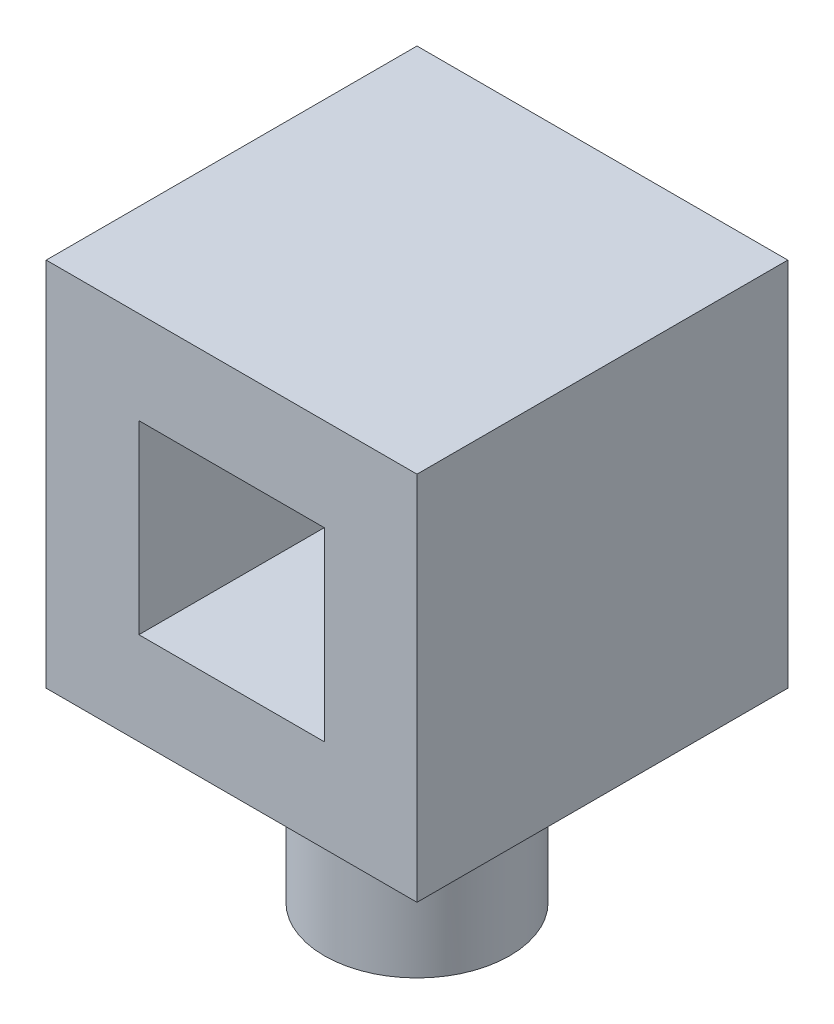
from build123d import *

# Parameters (mm, degrees)
SKETCH_1_W      = 20
SKETCH_1_H      = 20
SKETCH_1_W_2    = 10
SKETCH_1_H_2    = 10
EXTRUDE_1_DEPTH = 10
SKETCH_2_R      = 5
EXTRUDE_2_DEPTH = 10


with BuildPart() as part:
    # 草图1 → 凸台-拉伸1 (new, symmetric)
    with BuildSketch(Plane.XY):
        with Locations((5, 5)):
            Rectangle(SKETCH_1_W, SKETCH_1_H)
        with Locations((5, 5)):
            Rectangle(SKETCH_1_W_2, SKETCH_1_H_2, mode=Mode.SUBTRACT)
    extrude(amount=EXTRUDE_1_DEPTH, both=True)

    # 草图2 → 凸台-拉伸2 (add)
    with BuildSketch(Plane.XZ.offset(5)):
        with Locations(Location((5, 0, 0), (0, 0, 90))):
            Circle(SKETCH_2_R)
    extrude(amount=EXTRUDE_2_DEPTH)


solid = part.part
